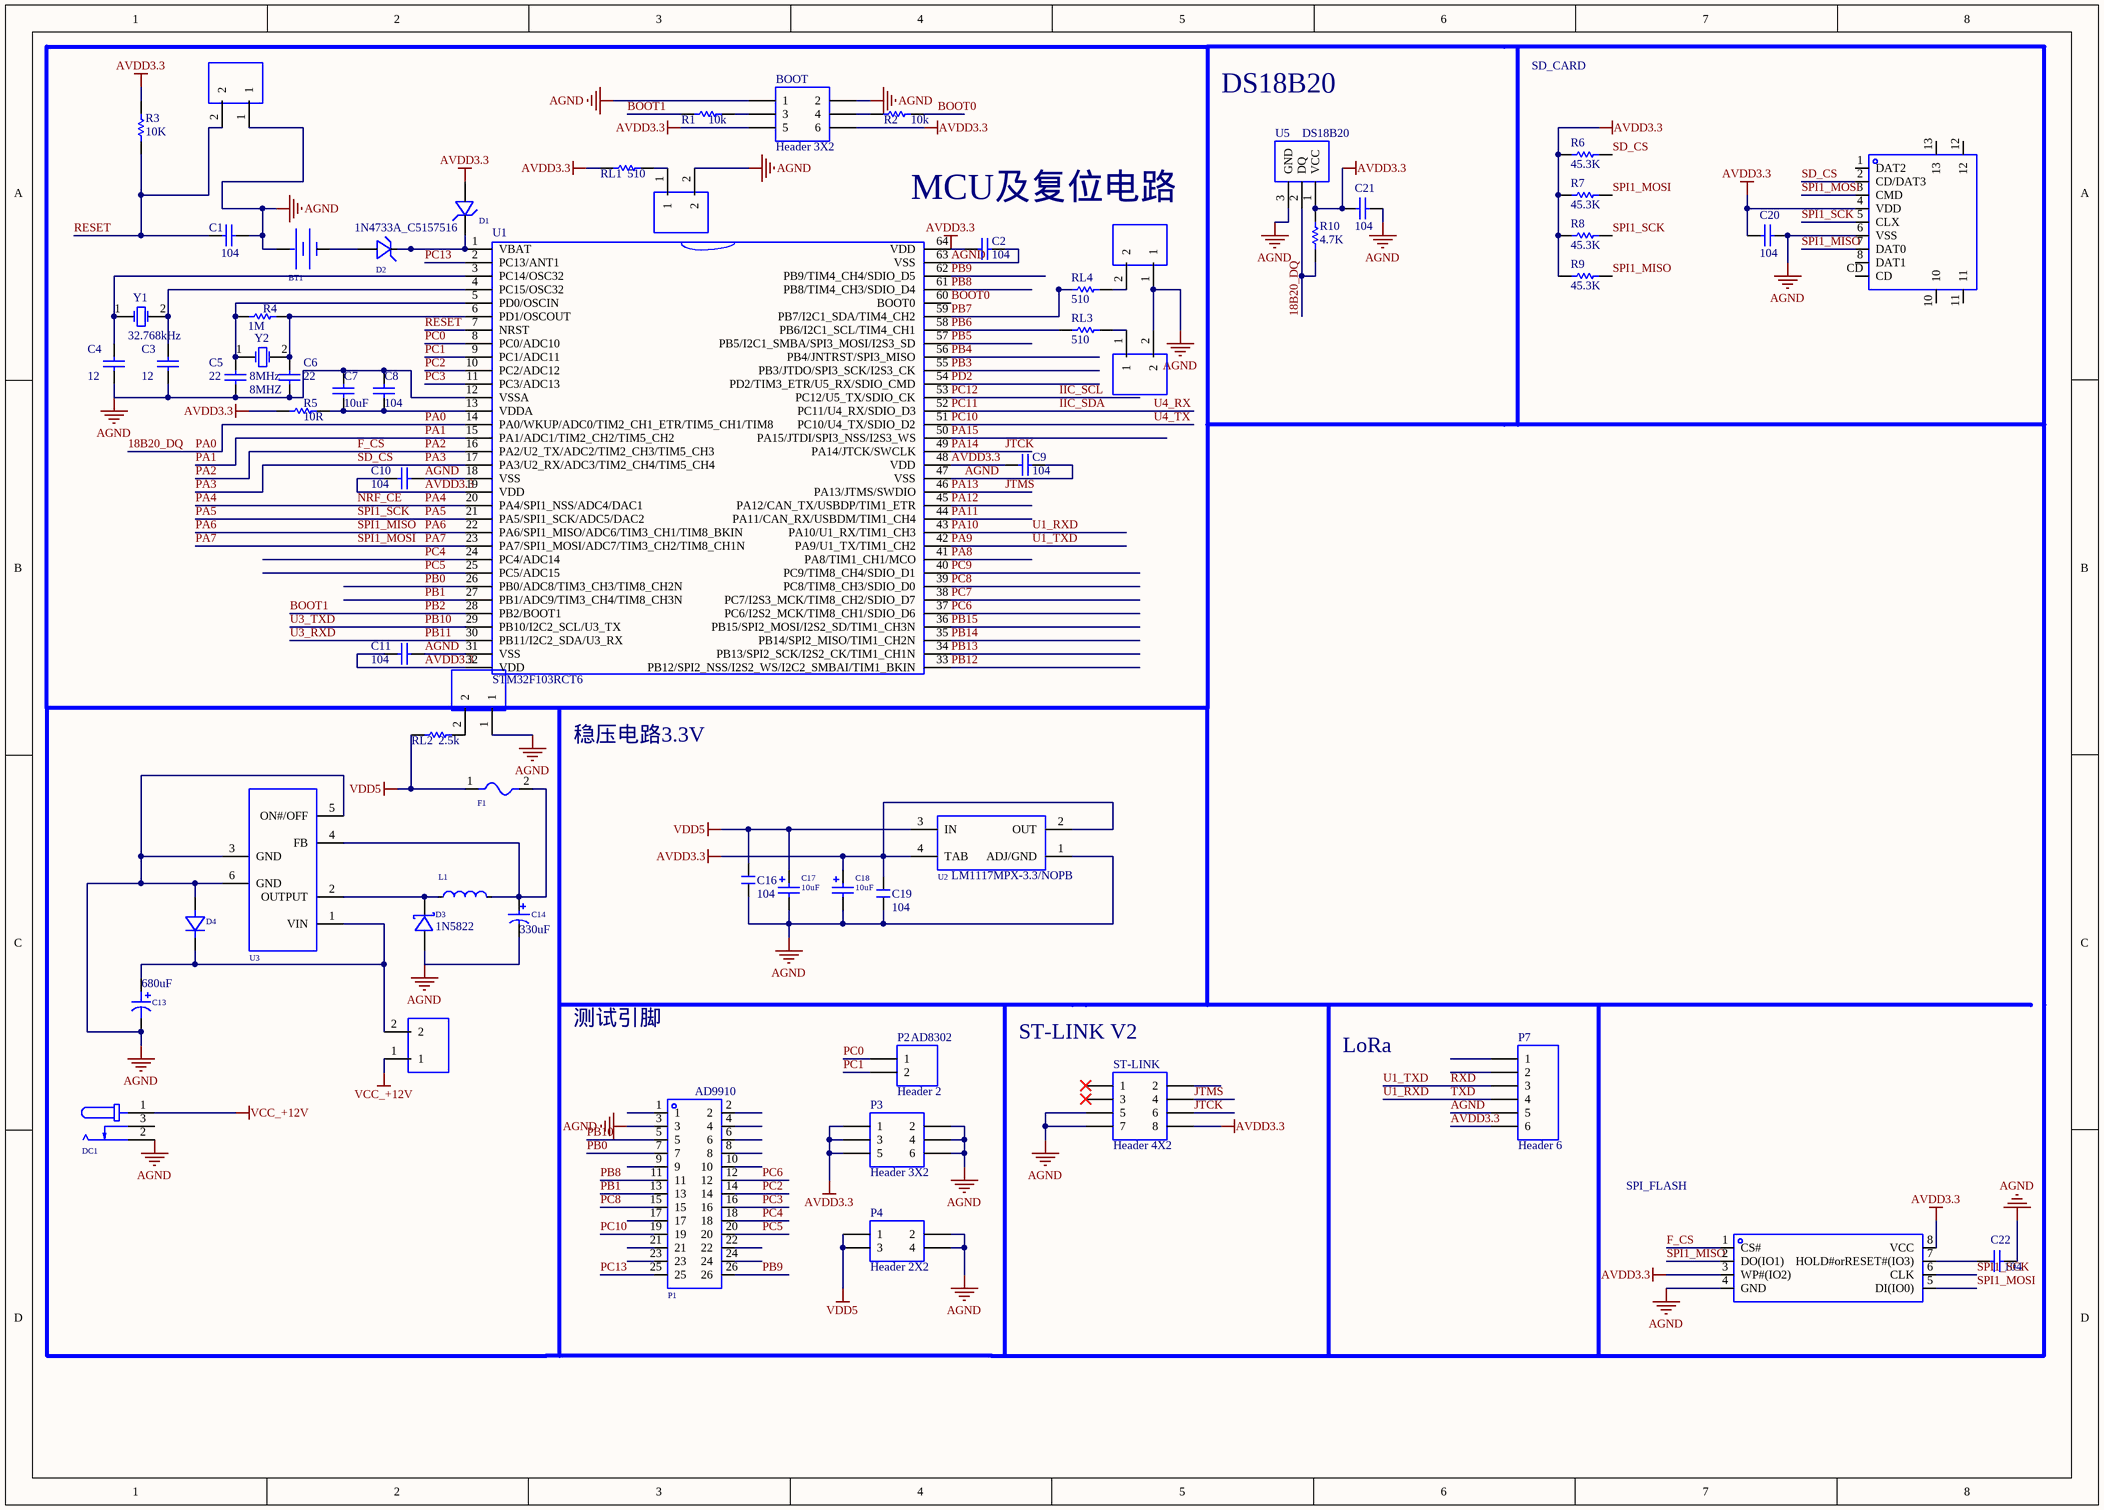
[diagram p0: MISC51485-3.schdoc]
# Altium project MISC51485-2.PrjPcb (part 2 of 2)
## Sheet MISC51485-3.schdoc: MISC51485 (continued)
### Parts (continued)
R1  10k  [R0603 - duplicate]
R2  10k  [R0603]
R3  10k  [R0603]
R4  1M  [R0603]
R5  10R  [R0603]
R6  Res  [RES[0603]]  (value not drawn)
R7  Res  [RES[0603]]  (value not drawn)
R8  Res  [RES[0603]]  (value not drawn)
R9  Res  [RES[0603]]  (value not drawn)
R10  Res  [RES[0603]]  (value not drawn)
RL1  330  [R0603 - duplicate]  (value not drawn)
RL2  330  [R0603 - duplicate]  (value not drawn)
RL3  330  [R0603 - duplicate]  (value not drawn)
RL4  330  [R0603 - duplicate]  (value not drawn)
ST-LINK  Header 4X2  [HDR2X4]
U1  STM32F103RCT6  [TQFP-64_L10.0-W10.0-P0.50-LS12.0-BL]
U2  LM1117MPX-3.3/NOPB  [SOT-223-3_L6.5-W3.4-P2.30-LS7.0-BR]
U3  LM2596SX-5.0/NOPB  [TO-263-5_L10.2-W8.9-P1.70-TL]  (value not drawn)
U5  DS18B20  [H2.54-1X3(RM)]
W25Q64  W25Q64JVSSIQ  [SOIC-8_L5.3-W5.3-P1.27-LS8.0-BL]  (value not drawn)
Y1  32.768kHz  [OSC-TH_BD2.0-P0.70-D0.3]
Y2  8MHz  [OSC-TH_L11.1-W4.7-P4.88]

### Blocks framed on the sheet
MCU及复位电路: BOOT BT1 C1-C11 D1 D2 P18-P21 P23 R1-R5 RL1 RL3 RL4 U1 Y1 Y2

### Nets
AGND: BOOT.1 BOOT.2 BT1.1(+) C1.2 C2.2 C3.1 C4.1 C5.1 C6.1 C7.2 C8.2 C9.2 C10.1 C11.1 C13.2 C14.2 C16.1 C17.2 C18.2 C19.1 C20.2 C21.2 C22.2 CARD.6(VSS) D3.1(A) D4.2(A) DC1.2 P1.3 P3.2 P3.4 P3.6 P4.2 P4.4 P7.5 P18.1 P19.2 P20.2 P21.1 P23.1 ST-LINK.5 ST-LINK.7 U1.12(VSSA) U1.18(VSS) U1.31(VSS) U1.47(VSS) U1.63(VSS) U2.1(ADJ/GND) U3.3(GND) U3.5(ON#/OFF) U3.6(GND) U5.3(GND) W25Q64.4(GND)
AVDD3.3: BOOT.5 BOOT.6 C2.1 C9.1 C10.2 C11.2 C18.1 C19.2 C20.1 C21.1 CARD.4(VDD) D1.2(A) P3.1 P3.3 P3.5 P7.6 R3.2 R5.2 R6.1 R7.1 R8.1 R9.1 R10.2 RL1.1 ST-LINK.8 U1.19(VDD) U1.32(VDD) U1.48(VDD) U1.64(VDD) U2.2(OUT) U2.4(TAB) U5.1(VCC) W25Q64.3(WP#(IO2)) W25Q64.8(VCC)
VCC_+12V: DC1.1 P22.1
VDD5: C16.2 C17.1 F1.1 P4.1 P4.3 RL2.1 U2.3(IN)
18B20_DQ: R10.1 U1.14(PA0/WKUP/ADC0/TIM2_CH1_ETR/TIM5_CH1/TIM8) U5.2(DQ)  [also labelled PA0]
BOOT0: R2.2 U1.60(BOOT0)
BOOT1: R1.1 U1.28(PB2/BOOT1)  [also labelled PB2]
F_CS: U1.16(PA2/U2_TX/ADC2/TIM2_CH3/TIM5_CH3) W25Q64.1(CS#)  [also labelled PA2]
IIC_SCL: U1.53(PC12/U5_TX/SDIO_CK)  [also labelled PC12]
IIC_SDA: U1.52(PC11/U4_RX/SDIO_D3)  [also labelled PC11, U4_RX]
JTCK: ST-LINK.6 U1.49(PA14/JTCK/SWCLK)  [also labelled PA14]
JTMS: ST-LINK.4 U1.46(PA13/JTMS/SWDIO)  [also labelled PA13]
NRF_CE: U1.20(PA4/SPI1_NSS/ADC4/DAC1)  [also labelled PA4]
PA1: U1.15(PA1/ADC1/TIM2_CH2/TIM5_CH2)
PA3: CARD.2(CD/DAT3) R6.2 U1.17(PA3/U2_RX/ADC3/TIM2_CH4/TIM5_CH4)  [also labelled SD_CS]
PA5: CARD.5(CLX) R8.2 U1.21(PA5/SPI1_SCK/ADC5/DAC2) W25Q64.6(CLK)  [also labelled SPI1_SCK]
PA6: CARD.7(DAT0) R9.2 U1.22(PA6/SPI1_MISO/ADC6/TIM3_CH1/TIM8_BKIN) W25Q64.2(DO(IO1))  [also labelled SPI1_MISO]
PA7: CARD.3(CMD) R7.2 U1.23(PA7/SPI1_MOSI/ADC7/TIM3_CH2/TIM8_CH1N) W25Q64.5(DI(IO0))  [also labelled SPI1_MOSI]
PA8: U1.41(PA8/TIM1_CH1/MCO)
PA9: P7.3 U1.42(PA9/U1_TX/TIM1_CH2)  [also labelled RXD, U1_TXD]
PA10: P7.4 U1.43(PA10/U1_RX/TIM1_CH3)  [also labelled TXD, U1_RXD]
PA11: U1.44(PA11/CAN_RX/USBDM/TIM1_CH4)
PA12: U1.45(PA12/CAN_TX/USBDP/TIM1_ETR)
PA15: U1.50(PA15/JTDI/SPI3_NSS/I2S3_WS)
PB0: P1.7 U1.26(PB0/ADC8/TIM3_CH3/TIM8_CH2N)
PB1: P1.13 U1.27(PB1/ADC9/TIM3_CH4/TIM8_CH3N)
PB3: U1.55(PB3/JTDO/SPI3_SCK/I2S3_CK)
PB4: U1.56(PB4/JNTRST/SPI3_MISO)
PB5: U1.57(PB5/I2C1_SMBA/SPI3_MOSI/I2S3_SD)
PB6: RL3.2 U1.58(PB6/I2C1_SCL/TIM4_CH1)
PB7: RL4.2 U1.59(PB7/I2C1_SDA/TIM4_CH2)
PB8: P1.11 U1.61(PB8/TIM4_CH3/SDIO_D4)
PB9: P1.26 U1.62(PB9/TIM4_CH4/SDIO_D5)
PB10: P1.5 U1.29(PB10/I2C2_SCL/U3_TX)  [also labelled U3_TXD]
PB11: U1.30(PB11/I2C2_SDA/U3_RX)  [also labelled U3_RXD]
PB12: U1.33(PB12/SPI2_NSS/I2S2_WS/I2C2_SMBAI/TIM1_BKIN)
PB13: U1.34(PB13/SPI2_SCK/I2S2_CK/TIM1_CH1N)
PB14: U1.35(PB14/SPI2_MISO/TIM1_CH2N)
PB15: U1.36(PB15/SPI2_MOSI/I2S2_SD/TIM1_CH3N)
PC0: P2.1 U1.8(PC0/ADC10)
PC1: P2.2 U1.9(PC1/ADC11)
PC2: P1.14 U1.10(PC2/ADC12)
PC3: P1.16 U1.11(PC3/ADC13)
PC4: P1.18 U1.24(PC4/ADC14)
PC5: P1.20 U1.25(PC5/ADC15)
PC6: P1.12 U1.37(PC6/I2S2_MCK/TIM8_CH1/SDIO_D6)
PC7: U1.38(PC7/I2S3_MCK/TIM8_CH2/SDIO_D7)
PC8: P1.15 U1.39(PC8/TIM8_CH3/SDIO_D0)
PC9: U1.40(PC9/TIM8_CH4/SDIO_D1)
PC10: P1.19 U1.51(PC10/U4_TX/SDIO_D2)  [also labelled U4_TX]
PC13: P1.25 U1.2(PC13/ANT1)
PD2: U1.54(PD2/TIM3_ETR/U5_RX/SDIO_CMD)
RESET: C1.1 P23.2 R3.1 U1.7(NRST)
NetBOOT_3: BOOT.3 R1.2
NetBOOT_4: BOOT.4 R2.1
NetBT1_2: BT1.2(-) D2.2(A)
NetC3_2: C3.2 U1.4(PC15/OSC32) Y1.2(OSC2)
NetC4_2: C4.2 U1.3(PC14/OSC32) Y1.1(OSC1)
NetC5_2: C5.2 R4.2 U1.5(PD0/OSCIN) Y2.1(OSC1)
NetC6_2: C6.2 R4.1 U1.6(PD1/OSCOUT) Y2.2(OSC2)
NetC7_1: C7.1 C8.1 R5.1 U1.13(VDDA)
NetC13_1: C13.1 D4.1(K) P22.2 U3.1(VIN)
NetC14_1: C14.1 F1.2 L1.2 U3.4(FB)
NetC22_1: C22.1 W25Q64.7(HOLD#orRESET#(IO3))
NetD1_1: D1.1(C) D2.1(C) U1.1(VBAT)
NetD3_2: D3.2(K) L1.1 U3.2(OUTPUT)
NetP18_2: P18.2 RL4.1
NetP19_1: P19.1 RL3.1
NetP20_1: P20.1 RL1.2
NetP21_2: P21.2 RL2.2

Not connected (* = marked no-connect by the designer): CARD 1(DAT2) 8(DAT1) 10 11 12 13 CD; DC1 3; P1 1 2 4 6 8 9 10 17 21 22 23 24; P7 1 2; ST-LINK 1* 2 3*

### Notes on the sheet
- DS18B20
- SD_CARD
- 稳压电路3.3V
- (near C13) 680uF
- (near C14) 330uF
- 测试引脚
- (near P2) AD8302
- (near ST-LINK) ST-LINK V2
- LoRa
- (near P1) AD9910
- SPI_FLASH

### Library data of the parts
BOOT = Header 3X2: Header, 3-Pin, Dual row; UniqueId: fb89199b69e6e72a; AddInBom: yes; Device: Header 3X2; LatestRevisionDate: 17-Jul-2002; LatestRevisionNote: Re-released for DXP Platform.; DesignItemID: Header 3X2; LibraryName: Miscellaneous Connectors; SymbolName: Header 3X2; FootprintName: HDR2X3; Publisher: Altium Limited
BT1 = BS-12-B3AA003: Manufacturer: MYOUNG(美阳); Add into BOM: yes; Connector Type: 电池底座; Battery Type: CR1220; UniqueId: 6f96c163600b442f; ModelId: 54ee14fdfc2a4013838c0af10e1f0cfd; Device: BS-12-B3AA003; LCSC Part Name: BS-12-B3AA003; Supplier Part: C964723; Manufacturer Part: BS-12-B3AA003; Supplier Footprint: SMD; JLCPCB Part Class: Extended Part; Datasheet: https://atta.szlcsc.com/upload/public/pdf/source/20201218/C964723_733B638E287393F86295A2A4DAE43C75.pdf; Supplier: LCSC; Convert to PCB: yes; Operating Temperature Range: -25℃~+85℃; DesignItemID: BS-12-B3AA003; LibraryName: BS-12-B3AA0031_BS-12-B3AA003.schdoc; SymbolName: BS-12-B3AA003; FootprintName: BAT-SMD_BS-12-B3AA011; ModelName: BAT-SMD_BS-12-B3AA011
C1 = 104: Origin Footprint: CAP[0805]; UniqueId: 5fb4f22ffcb6a001; SymbolName: Cap; AddInBom: yes; ModelId: fca5be93b99f4b5a9a2fd372d58c31d9; Device: 104; DesignItemID: Cap; LibraryName: Sean; Description: 104; FootprintName: C0603; ModelName: C0603
C2 = 104: Origin Footprint: CAP[0805]; UniqueId: 21d50210554cb61f; SymbolName: Cap; AddInBom: yes; ModelId: fca5be93b99f4b5a9a2fd372d58c31d9; Device: 104; DesignItemID: Cap; LibraryName: Sean; Description: 104; FootprintName: C0603; ModelName: C0603
C3 = 12pF: Origin Footprint: CAP[0805]; UniqueId: ec64484c8c07847f; SymbolName: Cap; AddInBom: yes; ModelId: fca5be93b99f4b5a9a2fd372d58c31d9; Device: 12pF; DesignItemID: Cap; LibraryName: Sean; Description: 12pF; FootprintName: C0603; ModelName: C0603
C4 = 12pF: Origin Footprint: CAP[0805]; UniqueId: 623e2bb2442f04df; SymbolName: Cap; AddInBom: yes; ModelId: fca5be93b99f4b5a9a2fd372d58c31d9; Device: 12pF; DesignItemID: Cap; LibraryName: Sean; Description: 12pF; FootprintName: C0603; ModelName: C0603
C5 = 22pF: Origin Footprint: CAP[0805]; UniqueId: 05d417a4d81547fc; SymbolName: Cap; AddInBom: yes; ModelId: fca5be93b99f4b5a9a2fd372d58c31d9; Device: 22pF; DesignItemID: Cap; LibraryName: Sean; Description: 22pF; FootprintName: C0603; ModelName: C0603
C6 = 22pF: Origin Footprint: CAP[0805]; UniqueId: d45ffe04e43665a4; SymbolName: Cap; AddInBom: yes; ModelId: fca5be93b99f4b5a9a2fd372d58c31d9; Device: 22pF; DesignItemID: Cap; LibraryName: Sean; Description: 22pF; FootprintName: C0603; ModelName: C0603
C7 = 10uF: Origin Footprint: CAP[0805]; OriginFootprint 2: CAP[1206]; UniqueId: 3007ca2539a35480; SymbolName: Cap; AddInBom: yes; ModelId: fca5be93b99f4b5a9a2fd372d58c31d9; Device: 10uF; DesignItemID: Cap; LibraryName: Sean; Description: 10uF; FootprintName: C0603; ModelName: C0603
C8 = 104: Origin Footprint: CAP[0805]; UniqueId: 878ab3ab0cce2757; SymbolName: Cap; AddInBom: yes; ModelId: fca5be93b99f4b5a9a2fd372d58c31d9; Device: 104; DesignItemID: Cap; LibraryName: Sean; Description: 104; FootprintName: C0603; ModelName: C0603
C9 = 104: Origin Footprint: CAP[0805]; UniqueId: 60e6893b044e2f17; SymbolName: Cap; AddInBom: yes; ModelId: fca5be93b99f4b5a9a2fd372d58c31d9; Device: 104; DesignItemID: Cap; LibraryName: Sean; Description: 104; FootprintName: C0603; ModelName: C0603
C10 = 104: Origin Footprint: CAP[0805]; UniqueId: c1764753ee6525b4; SymbolName: Cap; AddInBom: yes; ModelId: fca5be93b99f4b5a9a2fd372d58c31d9; Device: 104; DesignItemID: Cap; LibraryName: Sean; Description: 104; FootprintName: C0603; ModelName: C0603
C11 = 104: Origin Footprint: CAP[0805]; UniqueId: b49c3108c5288e9f; SymbolName: Cap; AddInBom: yes; ModelId: fca5be93b99f4b5a9a2fd372d58c31d9; Device: 104; DesignItemID: Cap; LibraryName: Sean; Description: 104; FootprintName: C0603; ModelName: C0603
C13 = GVM1V681M1010: 680uF; Manufacturer: HONOR(荣誉); Add into BOM: yes; Tolerance: ±20%; Rated Voltage: 35V; Ripple Current: 1.19A@120Hz; Equivalent Series Resistance(ESR): 60mΩ@120Hz; φD: 10mm; L: 10.2mm; Lifetime @ Temp: 5000hrs@105℃; UniqueId: 8d11a04c32f33369; ModelId: f51b16cd856a4d95baa34e209816f37c; Device: GVM1V681M1010; Supplier: LCSC; Supplier Part: C2980172; Manufacturer Part: GVM1V681M1010; Value: 680uF; JLCPCB Part Class: Extended Part; LCSC Part Name: 680uF ±20% 35V; Supplier Footprint: SMD,D10xL10.5mm; Datasheet: https://atta.szlcsc.com/upload/public/pdf/source/20220509/EB2A569F0F3393644DE07704993C28AA.pdf; Convert to PCB: yes; Operating Temperature: -55℃~+105℃; DesignItemID: GVM1V681M1010; LibraryName: Schlib1; SymbolName: GVM1V681M1010; FootprintName: CAP-SMD_BD10.0-L10.3-W10.3-LS10.9-FD; ModelName: CAP-SMD_BD10.0-L10.3-W10.3-LS10.9-FD
C14 = EEEFK1V331P: 330uF; Manufacturer: PANASONIC(松下); Add into BOM: yes; Tolerance: ±20%; Rated Voltage: 35V; Ripple Current: 637.5mA@120Hz; φD: 10mm; L: 10.5mm; Lifetime @ Temp: 5000hrs@105℃; UniqueId: c9f451b8b2c5f180; ModelId: b23815befd5e4172abc55cc8ac2654de; Device: EEEFK1V331P; Supplier: LCSC; Manufacturer Part: EEEFK1V331P; Value: 330uF; Supplier Part: C128512; JLCPCB Part Class: Extended Part; LCSC Part Name: 330uF ±20% 35V; Supplier Footprint: SMD,D10xL10.2mm; Datasheet: https://atta.szlcsc.com/upload/public/pdf/source/20180830/C242125_A6B570BC3E288FC2E03BFF90EF946F05.pdf; Convert to PCB: yes; Equivalent Series Resistance(ESR): -; Operating Temperature: -55℃~+105℃; DesignItemID: EEEFK1V331P; LibraryName: Schlib1; SymbolName: EEEFK1V331P; FootprintName: CAP-SMD_BD10.0-L10.3-W10.3-FD; ModelName: CAP-SMD_BD10.0-L10.3-W10.3-FD
C16 = 104_1: BOM名称: 无极性贴片电容; Origin Footprint: C 0201_L; OriginFootprint 2: C 0402_L; OriginFootprint 3: C 0603_L; OriginFootprint 4: C 0805_L; OriginFootprint 5: C 1206_L; OriginFootprint 6: C 1210_L; OriginFootprint 7: C 1808_L; OriginFootprint 8: C 1812_L; OriginFootprint 9: C 1825_L; OriginFootprint 10: C 2225_L; OriginFootprint 11: C 0201_M; OriginFootprint 12: C 0402_M; OriginFootprint 13: C 0603_M; OriginFootprint 14: C 0805_M; OriginFootprint 15: C 1206_M; OriginFootprint 16: C 1210_M; OriginFootprint 17: C 1808_M; OriginFootprint 18: C 1812_M; OriginFootprint 19: C 1825_M; OriginFootprint 20: C 2225_M; UniqueId: 6992a3033003bbbd; SymbolName: C; AddInBom: yes; ModelId: fca5be93b99f4b5a9a2fd372d58c31d9; Device: 104_1; DesignItemID: C; LibraryName: 3.1   - 电阻-电容-电感; Description: 104; FootprintName: C0603; ModelName: C0603
C17 = TAJA106K016RNJ: 10uF; Manufacturer: Kyocera AVX; Add into BOM: yes; Tolerance: ±10%; Rated Voltage: 16V; Equivalent Series Resistance(ESR): 3Ω@100kHz; UniqueId: 5e7964c847a08933; Device: TAJA106K016RNJ; LCSC Part Name: 10uF ±10% 16V; Supplier Part: C7171; Manufacturer Part: TAJA106K016RNJ; Supplier Footprint: CASE-A-3216; JLCPCB Part Class: Basic Part; Datasheet: https://atta.szlcsc.com/upload/public/pdf/source/20160107/1457707750344.pdf; Supplier: LCSC; Convert to PCB: yes; Operating Temperature: -55℃~+125℃; DesignItemID: TAJA106K016RNJ; LibraryName: TAJA106K016RNJ1_TAJA106K016RNJ.schdoc; SymbolName: TAJA106K016RNJ; FootprintName: CAP-SMD_L3.2-W1.6-RD-C7171
C18 = TAJA106K016RNJ: 10uF; Manufacturer: Kyocera AVX; Add into BOM: yes; Tolerance: ±10%; Rated Voltage: 16V; Equivalent Series Resistance(ESR): 3Ω@100kHz; UniqueId: 9b976857f3e39318; Device: TAJA106K016RNJ; LCSC Part Name: 10uF ±10% 16V; Supplier Part: C7171; Manufacturer Part: TAJA106K016RNJ; Supplier Footprint: CASE-A-3216; JLCPCB Part Class: Basic Part; Datasheet: https://atta.szlcsc.com/upload/public/pdf/source/20160107/1457707750344.pdf; Supplier: LCSC; Convert to PCB: yes; Operating Temperature: -55℃~+125℃; DesignItemID: TAJA106K016RNJ; LibraryName: Schlib1; SymbolName: TAJA106K016RNJ; FootprintName: CAP-SMD_L3.2-W1.6-RD-C7171
C19 = 104_1: BOM名称: 无极性贴片电容; Origin Footprint: C 0201_L; OriginFootprint 2: C 0402_L; OriginFootprint 3: C 0603_L; OriginFootprint 4: C 0805_L; OriginFootprint 5: C 1206_L; OriginFootprint 6: C 1210_L; OriginFootprint 7: C 1808_L; OriginFootprint 8: C 1812_L; OriginFootprint 9: C 1825_L; OriginFootprint 10: C 2225_L; OriginFootprint 11: C 0201_M; OriginFootprint 12: C 0402_M; OriginFootprint 13: C 0603_M; OriginFootprint 14: C 0805_M; OriginFootprint 15: C 1206_M; OriginFootprint 16: C 1210_M; OriginFootprint 17: C 1808_M; OriginFootprint 18: C 1812_M; OriginFootprint 19: C 1825_M; OriginFootprint 20: C 2225_M; UniqueId: 7dc0401965f49c44; SymbolName: C; AddInBom: yes; ModelId: fca5be93b99f4b5a9a2fd372d58c31d9; Device: 104_1; DesignItemID: C; LibraryName: 3.1   - 电阻-电容-电感; Description: 104; FootprintName: C0603; ModelName: C0603
C20 = Cap: 104; Origin Footprint: CAP[0805]; UniqueId: da3448d2adf90139; AddInBom: yes; OriginModelName: 0603_C; Device: Cap; DesignItemID: Cap; LibraryName: Sean; SymbolName: Cap; FootprintName: CAP[0603]
C21 = Cap: Origin Footprint: CAP[0805]; UniqueId: 8b38ef45c1644f88; AddInBom: yes; OriginModelName: 0603_C; Device: Cap; DesignItemID: Cap; LibraryName: Sean; Description: Cap; SymbolName: Cap; FootprintName: CAP[0603]
C22 = Cap: 104; Origin Footprint: CAP[0805]; UniqueId: 3f536f1ebce3e716; AddInBom: yes; OriginModelName: 0603_C; Device: Cap; DesignItemID: Cap; LibraryName: Sean; SymbolName: Cap; FootprintName: CAP[0603]
CARD = TF PUSH: Manufacturer: SHOU HAN(首韩); Add into BOM: yes; Card Type: MicroSD卡(TF卡); Connector Type: 卡座; Card Connection Mode: 自弹式; Maximum Body Height: 2mm; UniqueId: 8b068fab58f859d9; ModelId: 2d6270e77c9a43c6bb0aca962ba811a2; Device: TF PUSH; LCSC Part Name: 自弹式TF卡座 TF外焊式内存卡卡座; Supplier Part: C393941; Manufacturer Part: TF PUSH; Supplier Footprint: SMD; JLCPCB Part Class: Extended Part; Datasheet: https://atta.szlcsc.com/upload/public/pdf/source/20191011/C393941_0DDD896EE907FEB750D8B7B8982E2A67.pdf; Supplier: LCSC; Convert to PCB: yes; Operating Temperature Range: -20℃~+90℃; DesignItemID: TF PUSH; LibraryName: Schlib1; SymbolName: TF PUSH; FootprintName: TF-SMD_TF-PUSH; ModelName: TF-SMD_TF-PUSH
D1 = 1N4733A_C5157516: Manufacturer: LGE(鲁光); Add into BOM: yes; Diode Configuration: 独立式; Zener Voltage (Nom): 5.1V; Reverse Leakage Current (Ir): 5uA; Zener Voltage (Range): 4.85V~5.36V; Power Dissipation: 1W; Zener Impedance (Zzt): 7Ω; Tolerance: ±5%; UniqueId: 07a0d5848cd81316; ModelId: 20b412887349450cb9cb1509648d5b4d; Device: 1N4733A_C5157516; Supplier: LCSC; Supplier Part: C5157516; Manufacturer Part: 1N4733A; LCSC Part Name: 1N4733A; Supplier Footprint: DO-41; JLCPCB Part Class: Extended Part; Datasheet: https://atta.szlcsc.com/upload/public/pdf/source/20220902/F5B88186B80B648FAAEBF7A04A1CA013.pdf; Convert to PCB: yes; DesignItemID: 1N4733A_C5157516; LibraryName: 1N4733A_C51575161_1N4733A_C5157516.schdoc; SymbolName: 1N4733A_C5157516; FootprintName: DO-41_BD2.4-L4.7-P8.70-D0.9-RD; ModelName: DO-41_BD2.4-L4.7-P8.70-D0.9-RD
D2 = 1N4733A_C5157516: Manufacturer: LGE(鲁光); Add into BOM: yes; Diode Configuration: 独立式; Zener Voltage (Nom): 5.1V; Reverse Leakage Current (Ir): 5uA; Zener Voltage (Range): 4.85V~5.36V; Power Dissipation: 1W; Zener Impedance (Zzt): 7Ω; Tolerance: ±5%; UniqueId: fa5cd661465da5bc; ModelId: 20b412887349450cb9cb1509648d5b4d; Device: 1N4733A_C5157516; Supplier: LCSC; Supplier Part: C5157516; Manufacturer Part: 1N4733A; LCSC Part Name: 1N4733A; Supplier Footprint: DO-41; JLCPCB Part Class: Extended Part; Datasheet: https://atta.szlcsc.com/upload/public/pdf/source/20220902/F5B88186B80B648FAAEBF7A04A1CA013.pdf; Convert to PCB: yes; DesignItemID: 1N4733A_C5157516; LibraryName: 1N4733A_C51575161_1N4733A_C5157516.schdoc; SymbolName: 1N4733A_C5157516; FootprintName: DO-41_BD2.4-L4.7-P8.70-D0.9-RD; ModelName: DO-41_BD2.4-L4.7-P8.70-D0.9-RD
D3 = 1N5822: Manufacturer: MDD; Add into BOM: yes; Forward Voltage (Vf@If): 525mV@3A; Reverse Voltage (Vr): 40V; Average Rectified Current (Io): 3A; UniqueId: ce0e29427420bb9a; SymbolName: 1N5822_C2476; Device: 1N5822; Supplier: LCSC; Manufacturer Part: 1N5822; Supplier Part: C2476; JLCPCB Part Class: Extended Part; LCSC Part Name: 电压:40V 电流:3A; Supplier Footprint: DO-201AD; Datasheet: https://atta.szlcsc.com/upload/public/pdf/source/20230823/CE82667FA19214D7A9B56771CDBD17A6.pdf; Convert to PCB: yes; DesignItemID: 1N5822_C2476; LibraryName: Schlib1; FootprintName: DO-201AD_BD5.3-L8.4-P12.50-D1.4-FD
D4 = 1N4007_C727081: Manufacturer: TWGMC(台湾迪嘉); Manufacturer Part: 1N4007; Add into BOM: yes; Diode Configuration: 独立式; Forward Voltage (Vf@If): 1.1V@1A; Reverse Voltage (Vr): 1kV; Average Rectified Current (Io): 1A; Reverse Leakage Current: 5uA@1kV; UniqueId: 671e3575a93d22ee; ModelId: 5b53cc1b87a148cc9fa13125be89f948; Device: 1N4007_C727081; Supplier: LCSC; Supplier Part: C727081; JLCPCB Part Class: Extended Part; LCSC Part Name: 电压:1kV 电流:1A; Supplier Footprint: SMA(DO-214AC); Datasheet: https://atta.szlcsc.com/upload/public/pdf/source/20200828/C727079_3A05254382567072883400655AE0ED46.pdf; Convert to PCB: yes; DesignItemID: 1N4007_C727081; LibraryName: Schlib1; SymbolName: 1N4007_C727081; FootprintName: SMA_L4.3-W2.5-LS5.0-RD; ModelName: SMA_L4.3-W2.5-LS5.0-RD
DC1 = DC-005-20A_C136744: Manufacturer: 韩国韩荣; Add into BOM: yes; Inside Contact Diameter: 2mm; Outside Contact Diameter: 6.4mm; Current Rating (Max): 500mA; Voltage Rating (Max): 30V; UniqueId: 918354ff671956d3; ModelId: a72b9ca70a994526b1ddd7443b6051df; Device: DC-005-20A_C136744; LCSC Part Name: DC-005-20A  内芯2.0mm 全铜; Supplier Part: C136744; Manufacturer Part: DC-005-20A; Supplier Footprint: 插件; JLCPCB Part Class: Extended Part; Datasheet: https://atta.szlcsc.com/upload/public/pdf/source/20210810/D1FE451D887B1804F0660F580C4AD849.pdf; Supplier: LCSC; Convert to PCB: yes; DesignItemID: DC-005-20A_C136744; LibraryName: Schlib1; SymbolName: DC-005-20A_C136744; FootprintName: DC-IN-TH_DC-005-20A; ModelName: DC-IN-TH_DC-005-20A
F1 = BSMD1812-150-33V: Manufacturer: BHFUSE(佰宏); Add into BOM: yes; Operating Voltage (Max): 33V; Current Rating (Max): 40A; Hold Current: 1.5A; Trip Current: 3A; Power Dissipation: 1W; Resistance - Initial (Ri) (Min): 40mΩ; Resistance - Post Trip (R1) (Max): 160mΩ; Maximum Time to Trip: 500ms; UniqueId: 0327748d3d32b991; Device: BSMD1812-150-33V; Supplier: LCSC; Supplier Part: C883154; Manufacturer Part: BSMD1812-150-33V; JLCPCB Part Class: Extended Part; LCSC Part Name: 33V 1.5A 1812自恢复; Supplier Footprint: 1812; Datasheet: https://atta.szlcsc.com/upload/public/pdf/source/20230512/6ED7FF50F668B3AF958C55F12246A840.pdf; Convert to PCB: yes; Operating Temperature: -40℃~+85℃; DesignItemID: BSMD1812-150-33V; LibraryName: Schlib1; SymbolName: BSMD1812-150-33V; FootprintName: F1812
L1 = FXL0650-330-M: Manufacturer: cjiang(长江微电); Add into BOM: yes; Value: 33uH; Tolerance: ±20%; Rated Current: 2.3A; Saturation Current (Isat): 3A; DC Resistance (DCR): 190mΩ; Type: 一体成型电感; UniqueId: 2f42939b1ffc8518; Device: FXL0650-330-M; LCSC Part Name: 33uH ±20% 3A; Supplier Part: C475526; Manufacturer Part: FXL0650-330-M; Supplier Footprint: SMD,6.6x7mm; JLCPCB Part Class: Extended Part; Datasheet: https://atta.szlcsc.com/upload/public/pdf/source/20230516/677FF0B270D5BF5CC59B858CE23820C0.pdf; Supplier: LCSC; Convert to PCB: yes; DesignItemID: FXL0650-330-M; LibraryName: Schlib1; SymbolName: FXL0650-330-M; FootprintName: IND-SMD_L7.0-W6.6_FXL0650
P1 = X1270WV-2x13A-6TV01: Manufacturer: XKB Connectivity(中国星坤); Add into BOM: yes; UniqueId: f88e3064cb77b82c; SymbolName: IDC26; Device: X1270WV-2x13A-6TV01; LCSC Part Name: X1270WV-2x13A-6TV01; Supplier Part: C2962229; Manufacturer Part: X1270WV-2x13A-6TV01; Supplier Footprint: 插件,P=1.27mm; JLCPCB Part Class: Extended Part; Datasheet: https://atta.szlcsc.com/upload/public/pdf/source/20220119/2B69FB5CD1159548117BE170C9531B28.pdf; Supplier: LCSC; Convert to PCB: yes; Connector Type: -; Pitch: -; Current Rating (Max): -; Voltage Rating (Max): -; Holder Type: -; Row Spacing: -; Number of Rows: -; Pin Number in each Row: -; Contact Material: -; Contact Plating: -; Operating Temperature Range: -; Soldering Temperature(Max): -; DesignItemID: IDC26; LibraryName: Schlib1; FootprintName: IDC-TH_X1270WV-2X13A-6TV01
P2 = Header 2: Header, 2-Pin; UniqueId: ddb6c992c6045fb8; AddInBom: yes; Device: Header 2; LatestRevisionDate: 17-Jul-2002; LatestRevisionNote: Re-released for DXP Platform.; DesignItemID: Header 2; LibraryName: Miscellaneous Connectors; SymbolName: Header 2; FootprintName: HDR1X2; Publisher: Altium Limited
P3 = Header 3X2_1: Header, 3-Pin, Dual row; UniqueId: 10472a1c2ba3b044; AddInBom: yes; Device: Header 3X2_1; LatestRevisionDate: 17-Jul-2002; LatestRevisionNote: Re-released for DXP Platform.; DesignItemID: Header 3X2; LibraryName: Miscellaneous Connectors; SymbolName: Header 3X2; FootprintName: HDR2X3; Publisher: Altium Limited
P4 = Header 2X2: Header, 2-Pin, Dual row; UniqueId: 28b6bd94bccb65c1; AddInBom: yes; Device: Header 2X2; LatestRevisionDate: 17-Jul-2002; LatestRevisionNote: Re-released for DXP Platform.; DesignItemID: Header 2X2; LibraryName: Miscellaneous Connectors; SymbolName: Header 2X2; FootprintName: HDR2X2; Publisher: Altium Limited
P7 = Header 6: Header, 6-Pin; UniqueId: 6da615b7b85b0af3; AddInBom: yes; Device: Header 6; LatestRevisionDate: 17-Jul-2002; LatestRevisionNote: Re-released for DXP Platform.; DesignItemID: Header 6; LibraryName: Miscellaneous Connectors; SymbolName: Header 6; FootprintName: HDR1X6; Publisher: Altium Limited
P18 = WJ126V-5.0-2P: Manufacturer: KANGNEX(康奈克斯电气); Add into BOM: yes; Structure: 1x2P; Pitch: 5mm; Current Rating (Max): 18A; Voltage Rating (Max): 250V; Wire Gauge - AWG: 14~26; Wire Gauge - mm2: 2.5; Number of PINs Per Row: 2; UniqueId: 6c417fe5860076ce; SymbolName: 螺钉接线端子; Device: WJ126V-5.0-2P; Supplier: LCSC; Manufacturer Part: WJ126V-5.0-2P; Supplier Part: C8404; JLCPCB Part Class: Extended Part; LCSC Part Name: 5mm 1x2P 排数:1 每排P数:2 直插; Supplier Footprint: 插件,P=5mm; Datasheet: https://atta.szlcsc.com/upload/public/pdf/source/20191225/C8404_8F52D87DF851D149A4DEA9BD9FA83F9A.pdf; Convert to PCB: yes; Color: 绿色; Mounting Style: 直插; Number of Pins: 2P; Number of Rows: 1; Operating Temperature Range: -40℃~+105℃; DesignItemID: 螺钉接线端子; LibraryName: Schlib1; FootprintName: CONN-TH_WJ126V-5.0-2P
P19 = WJ126V-5.0-2P: Manufacturer: KANGNEX(康奈克斯电气); Add into BOM: yes; Structure: 1x2P; Pitch: 5mm; Current Rating (Max): 18A; Voltage Rating (Max): 250V; Wire Gauge - AWG: 14~26; Wire Gauge - mm2: 2.5; Number of PINs Per Row: 2; UniqueId: eac4bcba2edc5b91; SymbolName: 螺钉接线端子; Device: WJ126V-5.0-2P; Supplier: LCSC; Manufacturer Part: WJ126V-5.0-2P; Supplier Part: C8404; JLCPCB Part Class: Extended Part; LCSC Part Name: 5mm 1x2P 排数:1 每排P数:2 直插; Supplier Footprint: 插件,P=5mm; Datasheet: https://atta.szlcsc.com/upload/public/pdf/source/20191225/C8404_8F52D87DF851D149A4DEA9BD9FA83F9A.pdf; Convert to PCB: yes; Color: 绿色; Mounting Style: 直插; Number of Pins: 2P; Number of Rows: 1; Operating Temperature Range: -40℃~+105℃; DesignItemID: 螺钉接线端子; LibraryName: Schlib1; FootprintName: CONN-TH_WJ126V-5.0-2P
P20 = WJ126V-5.0-2P: Manufacturer: KANGNEX(康奈克斯电气); Add into BOM: yes; Structure: 1x2P; Pitch: 5mm; Current Rating (Max): 18A; Voltage Rating (Max): 250V; Wire Gauge - AWG: 14~26; Wire Gauge - mm2: 2.5; Number of PINs Per Row: 2; UniqueId: 9a9a53a3b7447df6; SymbolName: 螺钉接线端子; Device: WJ126V-5.0-2P; Supplier: LCSC; Manufacturer Part: WJ126V-5.0-2P; Supplier Part: C8404; JLCPCB Part Class: Extended Part; LCSC Part Name: 5mm 1x2P 排数:1 每排P数:2 直插; Supplier Footprint: 插件,P=5mm; Datasheet: https://atta.szlcsc.com/upload/public/pdf/source/20191225/C8404_8F52D87DF851D149A4DEA9BD9FA83F9A.pdf; Convert to PCB: yes; Color: 绿色; Mounting Style: 直插; Number of Pins: 2P; Number of Rows: 1; Operating Temperature Range: -40℃~+105℃; DesignItemID: 螺钉接线端子; LibraryName: Schlib1; FootprintName: CONN-TH_WJ126V-5.0-2P
P21 = WJ126V-5.0-2P: Manufacturer: KANGNEX(康奈克斯电气); Add into BOM: yes; Structure: 1x2P; Pitch: 5mm; Current Rating (Max): 18A; Voltage Rating (Max): 250V; Wire Gauge - AWG: 14~26; Wire Gauge - mm2: 2.5; Number of PINs Per Row: 2; UniqueId: c4d61bc3dce100d4; SymbolName: 螺钉接线端子; Device: WJ126V-5.0-2P; Supplier: LCSC; Manufacturer Part: WJ126V-5.0-2P; Supplier Part: C8404; JLCPCB Part Class: Extended Part; LCSC Part Name: 5mm 1x2P 排数:1 每排P数:2 直插; Supplier Footprint: 插件,P=5mm; Datasheet: https://atta.szlcsc.com/upload/public/pdf/source/20191225/C8404_8F52D87DF851D149A4DEA9BD9FA83F9A.pdf; Convert to PCB: yes; Color: 绿色; Mounting Style: 直插; Number of Pins: 2P; Number of Rows: 1; Operating Temperature Range: -40℃~+105℃; DesignItemID: 螺钉接线端子; LibraryName: Schlib1; FootprintName: CONN-TH_WJ126V-5.0-2P
P22 = WJ126V-5.0-2P_1: Manufacturer: KANGNEX(康奈克斯电气); Add into BOM: yes; Structure: 1x2P; Pitch: 5mm; Current Rating (Max): 18A; Voltage Rating (Max): 250V; Wire Gauge - AWG: 14~26; Wire Gauge - mm2: 2.5; Number of PINs Per Row: 2; UniqueId: 90eb7d180c052f31; SymbolName: 螺钉接线端子; Device: WJ126V-5.0-2P_1; Supplier: LCSC; Manufacturer Part: WJ126V-5.0-2P; Supplier Part: C8404; JLCPCB Part Class: Extended Part; LCSC Part Name: 5mm 1x2P 排数:1 每排P数:2 直插; Supplier Footprint: 插件,P=5mm; Datasheet: https://atta.szlcsc.com/upload/public/pdf/source/20191225/C8404_8F52D87DF851D149A4DEA9BD9FA83F9A.pdf; Convert to PCB: yes; Color: 绿色; Mounting Style: 直插; Number of Pins: 2P; Number of Rows: 1; Operating Temperature Range: -40℃~+105℃; DesignItemID: 螺钉接线端子; LibraryName: Schlib1; FootprintName: CONN-TH_WJ126V-5.0-2P
P23 = WJ126V-5.0-2P: Manufacturer: KANGNEX(康奈克斯电气); Add into BOM: yes; Structure: 1x2P; Pitch: 5mm; Current Rating (Max): 18A; Voltage Rating (Max): 250V; Wire Gauge - AWG: 14~26; Wire Gauge - mm2: 2.5; Number of PINs Per Row: 2; UniqueId: 557cfab0b7035923; SymbolName: 螺钉接线端子; Device: WJ126V-5.0-2P; Supplier: LCSC; Manufacturer Part: WJ126V-5.0-2P; Supplier Part: C8404; JLCPCB Part Class: Extended Part; LCSC Part Name: 5mm 1x2P 排数:1 每排P数:2 直插; Supplier Footprint: 插件,P=5mm; Datasheet: https://atta.szlcsc.com/upload/public/pdf/source/20191225/C8404_8F52D87DF851D149A4DEA9BD9FA83F9A.pdf; Convert to PCB: yes; Color: 绿色; Mounting Style: 直插; Number of Pins: 2P; Number of Rows: 1; Operating Temperature Range: -40℃~+105℃; DesignItemID: 螺钉接线端子; LibraryName: Schlib1; FootprintName: CONN-TH_WJ126V-5.0-2P
R1 = 10k_1: Origin Footprint: RES[0805]; OriginFootprint 2: Res; OriginFootprint 3: RES[0603]; UniqueId: 4e166b190d4de1c3; AddInBom: yes; Device: 10k_1; DesignItemID: Res; LibraryName: Sean; Description: 10K; SymbolName: Res; FootprintName: R0603 - duplicate
R2 = 10k: Origin Footprint: RES[0805]; OriginFootprint 2: Res; UniqueId: 06442d24ab060343; AddInBom: yes; ModelId: fc143cca1e79419f9cd78b61e9279f08; Device: 10k; DesignItemID: Res; LibraryName: Sean; Description: 10K; SymbolName: Res; FootprintName: R0603; ModelName: R0603
R3 = 10k: Origin Footprint: RES[0805]; OriginFootprint 2: Res; UniqueId: 6e26aea592918673; AddInBom: yes; ModelId: fc143cca1e79419f9cd78b61e9279f08; Device: 10k; DesignItemID: Res; LibraryName: Sean; Description: 10K; SymbolName: Res; FootprintName: R0603; ModelName: R0603
R4 = 1M: Res; Origin Footprint: RES[0805]; UniqueId: 49359f7360e76581; AddInBom: yes; ModelId: fc143cca1e79419f9cd78b61e9279f08; Device: 1M; OriginFootprint 2: Res; DesignItemID: Res; LibraryName: Sean; SymbolName: Res; FootprintName: R0603; ModelName: R0603
R5 = 10R: 10; Origin Footprint: RES[0805]; OriginFootprint 2: Res; UniqueId: 96bd3269827a783e; AddInBom: yes; ModelId: fc143cca1e79419f9cd78b61e9279f08; Device: 10R; DesignItemID: Res; LibraryName: Sean; SymbolName: Res; FootprintName: R0603; ModelName: R0603
R6 = Res: 45.3K; Origin Footprint: RES[0805]; UniqueId: c9a24d22ca7022dc; AddInBom: yes; OriginModelName: SW3dPS-0603 SMD Resistor; Device: Res; OriginFootprint 2: Res; DesignItemID: Res; LibraryName: Sean; SymbolName: Res; FootprintName: RES[0603]
R7 = Res: 45.3K; Origin Footprint: RES[0805]; UniqueId: 01f5c70ff2630ee7; AddInBom: yes; OriginModelName: SW3dPS-0603 SMD Resistor; Device: Res; OriginFootprint 2: Res; DesignItemID: Res; LibraryName: Sean; SymbolName: Res; FootprintName: RES[0603]
R8 = Res: 45.3K; Origin Footprint: RES[0805]; UniqueId: f0665cc51e401020; AddInBom: yes; OriginModelName: SW3dPS-0603 SMD Resistor; Device: Res; OriginFootprint 2: Res; DesignItemID: Res; LibraryName: Sean; SymbolName: Res; FootprintName: RES[0603]
R9 = Res: 45.3K; Origin Footprint: RES[0805]; UniqueId: 7a9d276dcc23a651; AddInBom: yes; OriginModelName: SW3dPS-0603 SMD Resistor; Device: Res; OriginFootprint 2: Res; DesignItemID: Res; LibraryName: Sean; SymbolName: Res; FootprintName: RES[0603]
R10 = Res: 4.7K; Origin Footprint: RES[0805]; UniqueId: 7663007c1f2bc029; AddInBom: yes; OriginModelName: SW3dPS-0603 SMD Resistor; Device: Res; OriginFootprint 2: Res; DesignItemID: Res; LibraryName: Sean; SymbolName: Res; FootprintName: RES[0603]
RL1 = 330: 510; Origin Footprint: RES[0805]; OriginFootprint 2: Res; OriginFootprint 3: RES[0603]; UniqueId: eb182b4c10ffa09b; AddInBom: yes; Device: 330; DesignItemID: Res; LibraryName: Sean; SymbolName: Res; FootprintName: R0603 - duplicate
RL2 = 330: 2.5K; Origin Footprint: RES[0805]; OriginFootprint 2: Res; OriginFootprint 3: RES[0603]; UniqueId: 29163dc8d5a5ba04; AddInBom: yes; Device: 330; DesignItemID: Res; LibraryName: Sean; SymbolName: Res; FootprintName: R0603 - duplicate
RL3 = 330: 510; Origin Footprint: RES[0805]; OriginFootprint 2: Res; OriginFootprint 3: RES[0603]; UniqueId: ce40cb1d1888fdab; AddInBom: yes; Device: 330; DesignItemID: Res; LibraryName: Sean; SymbolName: Res; FootprintName: R0603 - duplicate
RL4 = 330: 510; Origin Footprint: RES[0805]; OriginFootprint 2: Res; OriginFootprint 3: RES[0603]; UniqueId: 772c7d4909be14bd; AddInBom: yes; Device: 330; DesignItemID: Res; LibraryName: Sean; SymbolName: Res; FootprintName: R0603 - duplicate
ST-LINK = Header 4X2: Header, 4-Pin, Dual row; UniqueId: c23d0985ae090e0c; AddInBom: yes; Device: Header 4X2; LatestRevisionDate: 17-Jul-2002; LatestRevisionNote: Re-released for DXP Platform.; DesignItemID: Header 4X2; LibraryName: Miscellaneous Connectors; SymbolName: Header 4X2; FootprintName: HDR2X4; Publisher: Altium Limited
U1 = STM32F103RCT6: Origin Footprint: LQFP-64; UniqueId: 48a4a086d8c42a18; AddInBom: yes; Device: STM32F103RCT6; DesignItemID: STM32F103RCT6; LibraryName: Sean; SymbolName: STM32F103RCT6; FootprintName: TQFP-64_L10.0-W10.0-P0.50-LS12.0-BL
U2 = LM1117MPX-3.3/NOPB: Manufacturer: TI(德州仪器); Manufacturer Part: LM1117MP-5.0/NOPB; Add into BOM: yes; Current - Supply (Max): 10mA; Voltage - Input (Max): 15V; Voltage Dropout (Max): 1.2V @ 800mA; Output Current (Max): 800mA; Output Configuration: 正; Ripple Rejection (PSRR): 75dB(120Hz); Output Type: 固定; Number of Output Channels: 1; Voltage - Output (Fixed): 5V; UniqueId: d74c11912b695046; Device: LM1117MPX-3.3/NOPB; LCSC Part Name: LM1117MP-5.0/NOPB; Supplier Part: C131933; Supplier Footprint: SOT-223; JLCPCB Part Class: Extended Part; Datasheet: https://atta.szlcsc.com/upload/public/pdf/source/20170925/C131933_1506321508697990294.pdf; Supplier: LCSC; Convert to PCB: yes; Voltage - Output (adj): -; Quiescent Current (Iq): -; Operating Temperature: 0℃ ~ 125℃(TJ); Enabling feet: -; DesignItemID: LM1117MP-5.0/NOPB; LibraryName: Schlib1; SymbolName: LM1117MP-5.0/NOPB; FootprintName: SOT-223-3_L6.5-W3.4-P2.30-LS7.0-BR
U3 = LM2596SX-5.0/NOPB: Manufacturer: TI(德州仪器); Add into BOM: yes; Function: 降压型; Output Type: 固定; Input Voltage: 4.5V~40V; Output Voltage: 5V; Output Current (Max): 3A; Switching Frequency: 150kHz; Synchronous Rectification: 否; Number of Outputs: 1; Topology: 降压式; Switch tube (built-in/external): 内置; UniqueId: eac3f191c372887e; SymbolName: LM2596SX-5.0/NOPB_1; Device: LM2596SX-5.0/NOPB; LCSC Part Name: LM2596SX-5.0/NOPB; Supplier Part: C10002; Manufacturer Part: LM2596SX-5.0/NOPB; Supplier Footprint: TO-263-5; JLCPCB Part Class: Extended Part; Datasheet: https://www.ti.com/cn/lit/gpn/lm2596; Supplier: LCSC; Convert to PCB: yes; Operating Temperature: -40℃~+125℃@(TJ); DesignItemID: LM2596SX-5.0/NOPB_1; LibraryName: Schlib1; FootprintName: TO-263-5_L10.2-W8.9-P1.70-TL
U5 = DS18B20: UniqueId: 65fd737caad1a168; AddInBom: yes; OriginModelName: User Library-RM254_3pin; Device: DS18B20; DesignItemID: DS18B20; LibraryName: Sean; Description: DS18B20; SymbolName: DS18B20; FootprintName: H2.54-1X3(RM)
W25Q64 = W25Q64JVSSIQ: Manufacturer: WINBOND(华邦); Add into BOM: yes; UniqueId: e91f9b0dd8a76ba1; Device: W25Q64JVSSIQ; Supplier: LCSC; Supplier Part: C179171; Manufacturer Part: W25Q64JVSSIQ; JLCPCB Part Class: Extended Part; LCSC Part Name: W25Q64JVSSIQ; Supplier Footprint: SOIC-8-208mil; Datasheet: https://atta.szlcsc.com/upload/public/pdf/source/20191218/C179171_92C5C91D0324539EDD8F1160D2E79C0F.pdf; Convert to PCB: yes; DesignItemID: W25Q64JVSSIQ; LibraryName: W25Q64JVSSIQ_C1791711_W25Q64JVSSIQ_C179171.schdoc; SymbolName: W25Q64JVSSIQ; FootprintName: SOIC-8_L5.3-W5.3-P1.27-LS8.0-BL
Y1 = 32.768kHz: XTAL; OriginFootprint 2: OSC-TH_L11.1-W4.7-P4.88; UniqueId: c44a0eb1f1b20cbd; AddInBom: yes; Device: 32.768kHz; Origin Footprint: XTAL; DesignItemID: XTAL; LibraryName: Sean; SymbolName: XTAL; FootprintName: OSC-TH_BD2.0-P0.70-D0.3
Y2 = 8MHz: XTAL; UniqueId: ffd1e7cd05e9e4ae; AddInBom: yes; ModelId: f2ed30de83344a4b83b1c4b1b9fe1856; Device: 8MHz; Origin Footprint: XTAL; DesignItemID: XTAL; LibraryName: Sean; SymbolName: XTAL; FootprintName: OSC-TH_L11.1-W4.7-P4.88; ModelName: OSC-TH_L11.1-W4.7-P4.88

## Nets that join several sheets
AGND: MISC51485-4 (6 pins), MISC51485-3 (52 pins)
VDD5: MISC51485-4 (10 pins), MISC51485-3 (7 pins)
PA12: MISC51485-4 (P12.2), MISC51485-3 (U1.45)
PC0: MISC51485-4 (R22.1), MISC51485-3 (P2.1 U1.8)
PC1: MISC51485-4 (R26.1), MISC51485-3 (P2.2 U1.9)